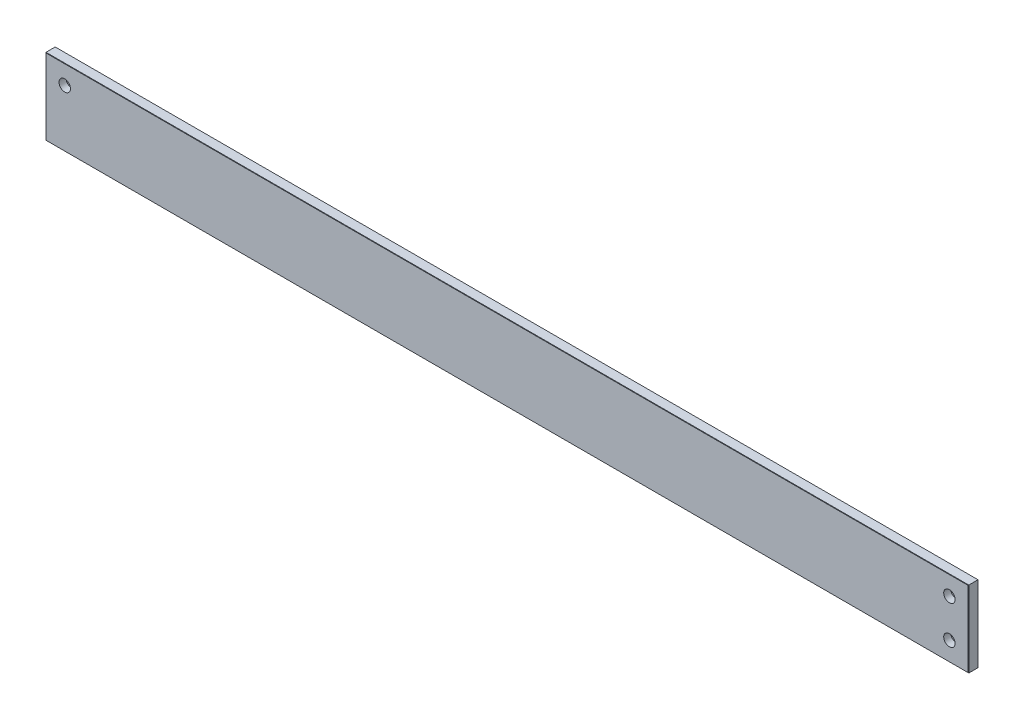
from build123d import *

# Parameters (mm, degrees)
SKETCH_1_W                = 1453
SKETCH_1_H                = 120
EXTRUDE_1_DEPTH           = 7.5
HOLE_WIZARD_1_D           = 11
HOLE_WIZARD_1_CBORE_D     = 18
HOLE_WIZARD_1_CBORE_DEPTH = 11
HOLE_WIZARD_2_D           = 11
HOLE_WIZARD_2_CBORE_D     = 18
HOLE_WIZARD_2_CBORE_DEPTH = 11
CHAMFER_1_SIZE            = 0.5


with BuildPart() as part:
    # 草图1 → 凸台-拉伸1 (new, symmetric)
    with BuildSketch(Plane.XY):
        Rectangle(SKETCH_1_W, SKETCH_1_H)
    extrude(amount=EXTRUDE_1_DEPTH, both=True)

    # 打孔尺寸(%根据)内六角圆柱头螺钉的类型1 (through all)
    with Locations(Plane(origin=(-696.5, 30, 7.5), x_dir=(1, 0, 0), z_dir=(0, 0, 1))):
        with Locations((0, 0)):
            CounterBoreHole(HOLE_WIZARD_1_D / 2, HOLE_WIZARD_1_CBORE_D / 2, HOLE_WIZARD_1_CBORE_DEPTH)

    # 打孔尺寸(%根据)内六角圆柱头螺钉的类型2 (through all)
    with Locations(Plane(origin=(696.5, 30, 7.5), x_dir=(1, 0, 0), z_dir=(0, 0, 1))):
        with Locations((0, 0), (0, -60)):
            CounterBoreHole(HOLE_WIZARD_2_D / 2, HOLE_WIZARD_2_CBORE_D / 2, HOLE_WIZARD_2_CBORE_DEPTH)

    # 倒角1
    chamfer_1_edges = [part.edges().sort_by_distance(p)[0] for p in [
        (-726.5, 0, 7.5),
        (0, -60, 7.5),
        (726.5, 0, 7.5),
        (0, 60, 7.5),
    ]]
    chamfer(chamfer_1_edges, length=CHAMFER_1_SIZE)


solid = part.part
